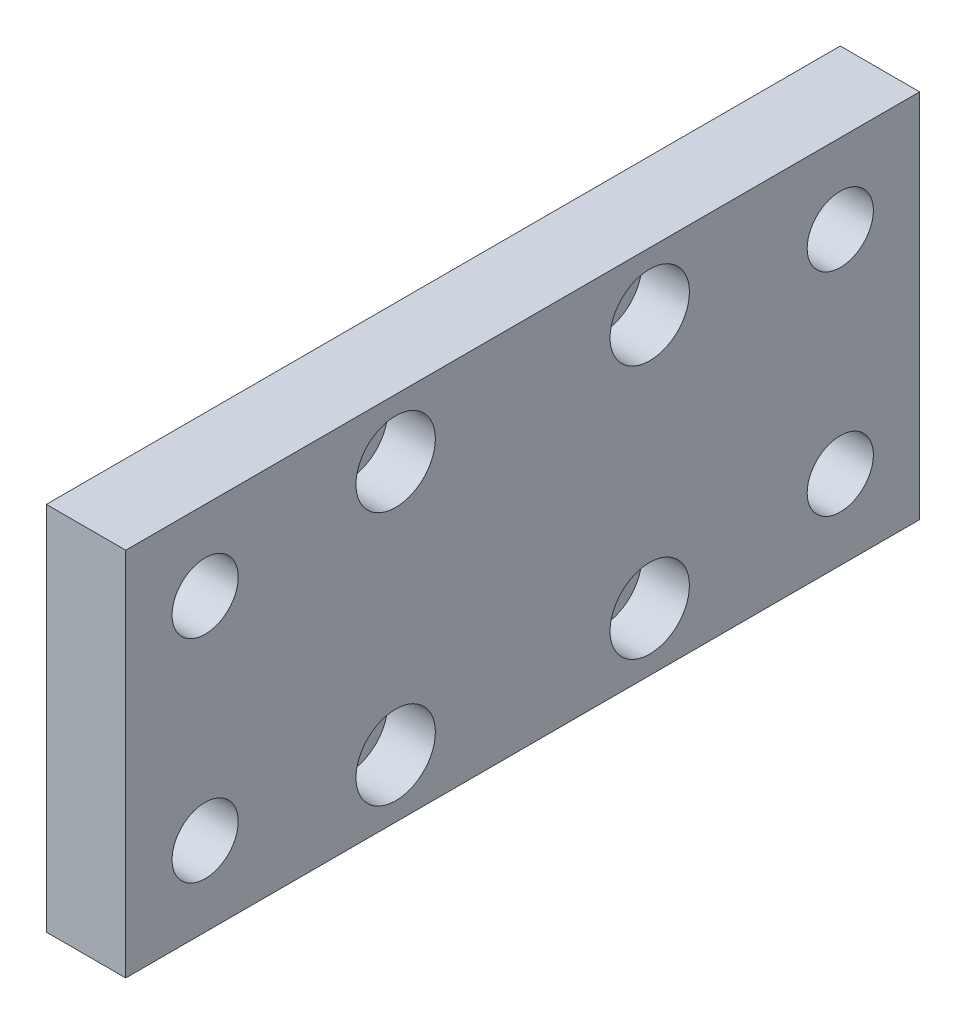
SolidWorks part; units mm, degrees
ref_plane "前视基准面" through (0, 0, 0) normal (0, 0, 1) x (1, 0, 0)
ref_plane "上视基准面" through (0, 0, 0) normal (0, 1, 0) x (1, 0, 0)
ref_plane "右视基准面" through (0, 0, 0) normal (1, 0, 0) x (0, 0, -1)
sketch "草图1" plane through (0, 0, 0) normal (1, 0, 0) x (0, 0, -1)
  line L1 (-75, 35) -> (75, 35)
  line L2 (-75, 35) -> (-75, -35)
  line L3 (-75, -35) -> (75, -35)
  line L4 (75, 35) -> (75, -35)
  line L5 (-75, 35) -> (75, -35) construction
  line L6 (-75, -35) -> (75, 35) construction
  point P0 (0, 0)
  dimension "D1" = 150
  dimension "D2" = 70
extrude "凸台-拉伸1" add sketch "草图1" along normal blind 15
hole_wizard "打孔尺寸(%根据)内六角圆柱头螺钉的类型1" positions "草图2" profile "草图3" counterbore size "M8" standard "GB" end condition through all
sketch "草图2" plane through (15, 0, 0) normal (1, 0, 0) x (0, 0, -1)
  line L0 (0, 84.4137) -> (0, 0) construction
  line L1 (0, 0) -> (71.8929, 0) construction
  point P0 (-24, 24)
  point P2 (24, 24)
  point P4 (-24, -24)
  point P6 (24, -24)
  dimension "D1" = 48
  dimension "D2" = 48
sketch "草图3" plane through (15, 24, 24) normal (0, 1, 0) x (0, 0, -1)
  line L0 (0, 0) -> (0, 15)
  line L1 (0, 15) -> (4.5, 15)
  line L3 (4.5, 15) -> (4.5, 9)
  line L4 (4.5, 9) -> (7.5, 9)
  line L5 (7.5, 9) -> (7.5, 0)
  line L7 (7.5, 0) -> (0, 0)
  line L11 (0, -6.35) -> (0, 107.95) construction
  dimension "通孔孔直径" = 9
  dimension "通孔孔深度" = 15
  dimension "柱形沉头孔直径" = 15
  dimension "柱形沉头孔深度" = 9
hole_wizard "Ø12.5 (12.5) 直径孔1" positions "草图4" profile "草图5" hole size "Ø12.5" standard "GB" end condition through all
sketch "草图4" plane through (0, 0, 0) normal (-1, 0, 0) x (0, 0, 1)
  line L0 (0, 98.291) -> (0, 0) construction
  line L1 (0, 0) -> (147.9622, 0) construction
  point P0 (-60, 20)
  point P2 (-60, -20)
  point P4 (60, 20)
  point P6 (60, -20)
  dimension "D1" = 120
  dimension "D2" = 40
sketch "草图5" plane through (0, 20, -60) normal (0, 1, 0) x (0, 0, 1)
  line L0 (0, 0) -> (0, 15)
  line L1 (0, 15) -> (6.25, 15)
  line L2 (6.25, 15) -> (6.25, 0)
  line L5 (6.25, 0) -> (0, 0)
  line L11 (0, -6.35) -> (0, 107.95) construction
  dimension "通孔孔直径" = 12.5
  dimension "通孔孔深度" = 15
